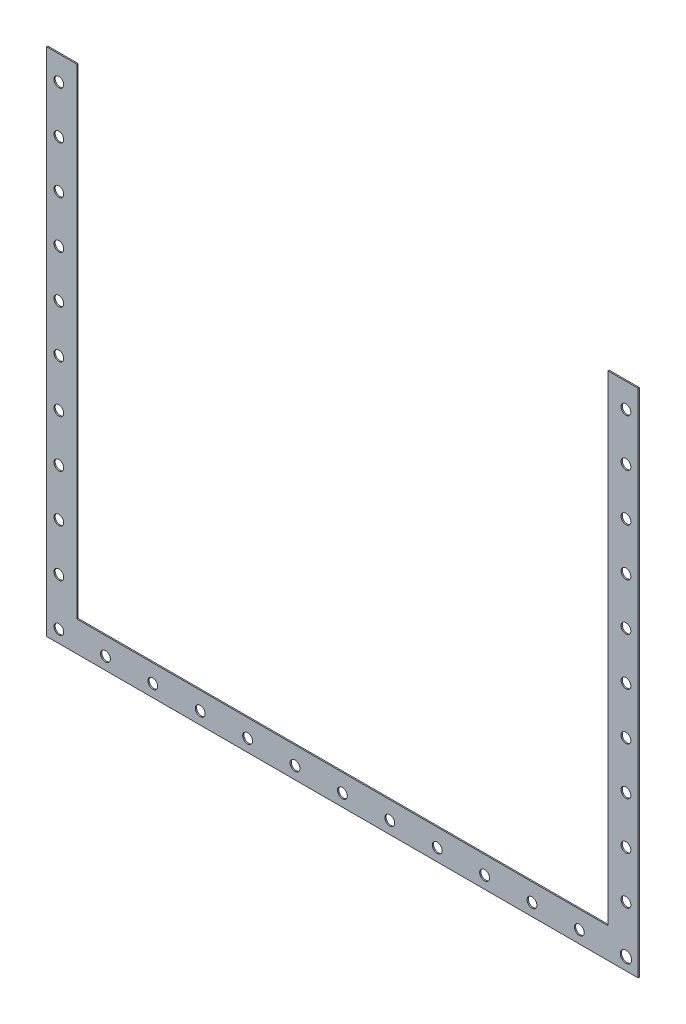
SolidWorks part; units mm, degrees
ref_plane "Front" through (0, 0, 0) normal (0, 0, 1) x (1, 0, 0)
ref_plane "Top" through (0, 0, 0) normal (0, 1, 0) x (1, 0, 0)
ref_plane "Right" through (0, 0, 0) normal (1, 0, 0) x (0, 0, -1)
sketch "Sketch1" plane through (0, 0, 0) normal (0, 0, 1) x (1, 0, 0)
  line L0 (-66.1787, 64.3057) -> (-66.1787, -1185.6943)
  line L1 (-66.1787, -1185.6943) -> (1381.8213, -1185.6943)
  line L2 (1381.8213, -1185.6943) -> (1381.8213, 64.3057)
  line L3 (7.8213, 64.3057) -> (7.8213, -1111.6943)
  line L4 (7.8213, -1111.6943) -> (1307.8213, -1111.6943)
  line L5 (1307.8213, -1111.6943) -> (1307.8213, 64.3057)
  line L6 (-66.1787, 64.3057) -> (7.8213, 64.3057)
  line L7 (1307.8213, 64.3057) -> (1381.8213, 64.3057)
  line L8 (1381.8213, 64.3057) -> (1384.4034, 64.9887)
  line L9 (657.8213, -1185.6943) -> (657.8213, -227.6943) construction
  circle A0 centre (-36.1787, 4.3057) radius 12
  circle A1 centre (-36.1787, -111.6943) radius 12
  circle A2 centre (-36.1787, -227.6943) radius 12
  circle A3 centre (-36.1787, -343.6943) radius 12
  circle A4 centre (-36.1787, -459.6943) radius 12
  circle A5 centre (-36.1787, -575.6943) radius 12
  circle A6 centre (-36.1787, -691.6943) radius 12
  circle A7 centre (-36.1787, -807.6943) radius 12
  circle A8 centre (-36.1787, -923.6943) radius 12
  circle A9 centre (-36.1787, -1039.6943) radius 12
  circle A10 centre (-36.1787, -1155.6943) radius 12
  circle A11 centre (77.8213, -1155.6943) radius 12
  circle A12 centre (193.8213, -1155.6943) radius 12
  circle A13 centre (309.8213, -1155.6943) radius 12
  circle A14 centre (425.8213, -1155.6943) radius 12
  circle A15 centre (541.8213, -1155.6943) radius 12
  circle A16 centre (657.8213, -1155.6943) radius 12
  circle A17 centre (773.8213, -1155.6943) radius 12
  circle A18 centre (889.8213, -1155.6943) radius 12
  circle A19 centre (1005.8213, -1155.6943) radius 12
  circle A20 centre (1121.8213, -1155.6943) radius 12
  circle A21 centre (1237.8213, -1155.6943) radius 12
  circle A22 centre (1351.8213, -1155.6943) radius 13.8489
  circle A23 centre (1351.8213, -1039.6943) radius 12
  circle A24 centre (1351.8213, -923.6943) radius 12
  circle A25 centre (1351.8213, -807.6943) radius 12
  circle A26 centre (1351.8213, -691.6943) radius 12
  circle A27 centre (1351.8213, -575.6943) radius 12
  circle A28 centre (1351.8213, -459.6943) radius 12
  circle A29 centre (1351.8213, -343.6943) radius 12
  circle A30 centre (1351.8213, -227.6943) radius 12
  circle A31 centre (1351.8213, -111.6943) radius 12
  circle A32 centre (1351.8213, 4.3057) radius 12
  dimension "D2" = 60
  dimension "D4" = 30
  dimension "D5" = 114
  dimension "D7" = 114
  dimension "D8" = 30
  dimension "D9" = 30
  dimension "D1" = 74
  dimension "D3" = 11
  dimension "D6" = 11
extrude "Boss-Extrude1" add sketch "Sketch1" along normal blind 3 contours L1 L9 A16 L4 L3 L6 L0 A0 A1 A2 A3 A4 A5 A6 A7 A8 A9 A10 A11 A12 A13 A14 A15 | L9 L1 L2 L7 L5 L4 A16 A31 A29 A27 A25 A23 A22 A21 A20 A19 A18 A17 A24 A26 A28 A30 A32
equation "\"零件重量\"= IIF ( \"SW-质量\" > 100 , int ( \"SW-质量\" ) , \"SW-质量\" )"
